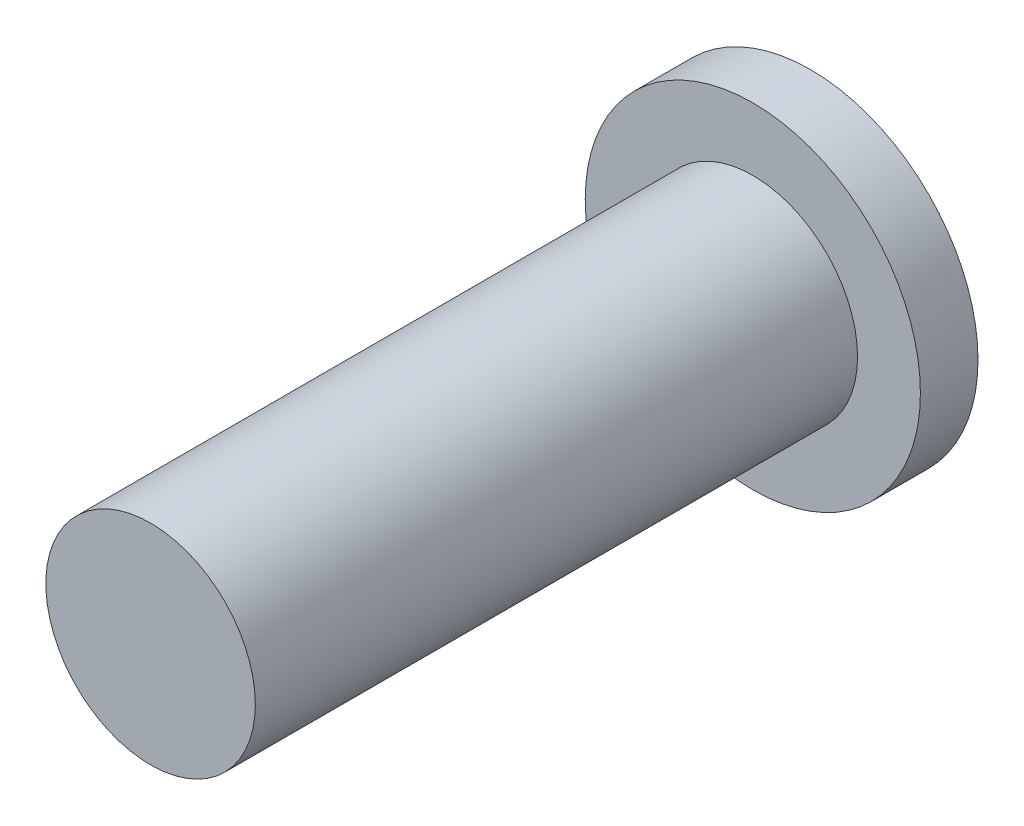
from build123d import *

# Parameters (mm, degrees)
SKETCH_1_R      = 10
EXTRUDE_1_DEPTH = 63
SKETCH_2_R      = 16
EXTRUDE_2_DEPTH = 5.5


with BuildPart() as part:
    # 草图1 → 凸台-拉伸1 (new body)
    with BuildSketch(Plane.XY):
        Circle(SKETCH_1_R)
    extrude(amount=EXTRUDE_1_DEPTH)

    # 草图2 → 凸台-拉伸2 (add)
    with BuildSketch(Plane.XY):
        Circle(SKETCH_2_R)
    extrude(amount=EXTRUDE_2_DEPTH)


solid = part.part
